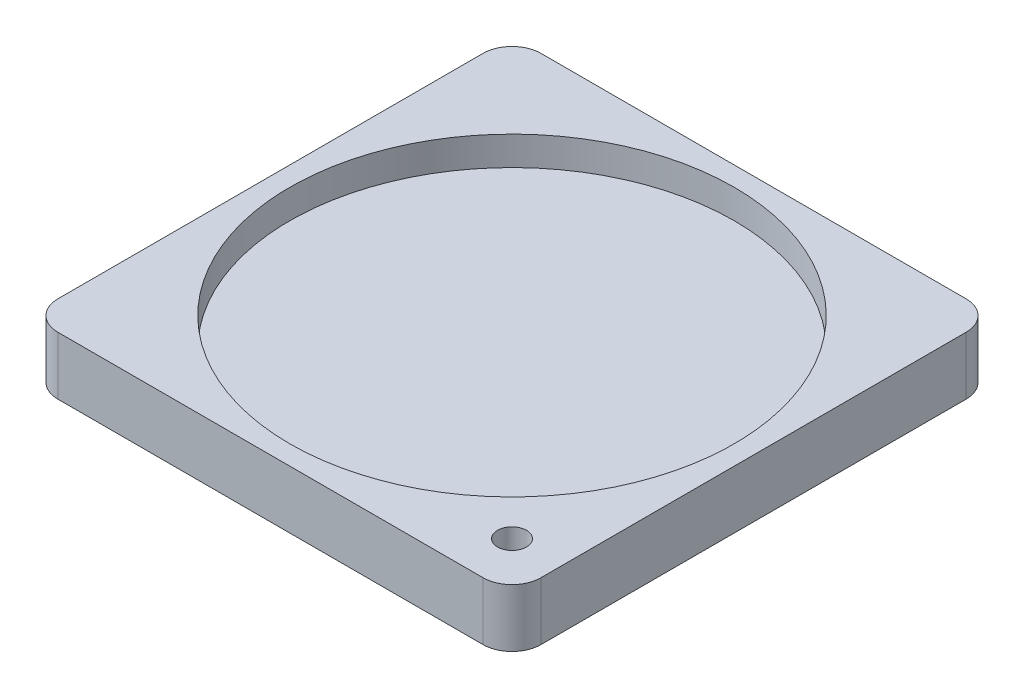
from build123d import *

# Parameters (mm, degrees)
SKETCH1_W           = 50
SKETCH1_H           = 50
BOSS_EXTRUDE1_DEPTH = 10
SKETCH2_R           = 23
CUT_EXTRUDE1_DEPTH  = 3
SKETCH3_R           = 1.5
CUT_EXTRUDE2_DEPTH  = 3
SKETCH4_W           = 50
SKETCH4_H           = 4
CUT_EXTRUDE3_DEPTH  = 76
FILLET1_R           = 3
SKETCH5_R           = 1.5
CUT_EXTRUDE4_DEPTH  = 1


with BuildPart() as part:
    # Sketch1 → Boss-Extrude1 (new body)
    with BuildSketch(Plane(origin=(0, 0, 0), x_dir=(1, 0, 0), z_dir=(0, 1, 0))):
        Rectangle(SKETCH1_W, SKETCH1_H)
    extrude(amount=BOSS_EXTRUDE1_DEPTH)

    # Sketch2 → Cut-Extrude1 (cut)
    with BuildSketch(Plane(origin=(0, 10, 0), x_dir=(1, 0, 0), z_dir=(0, 1, 0))):
        with Locations(Location((0, 0, 0), (0, 0, 270))):
            Circle(SKETCH2_R)
    extrude(amount=-CUT_EXTRUDE1_DEPTH, mode=Mode.SUBTRACT)

    # Sketch3 → Cut-Extrude2 (cut)
    with BuildSketch(Plane(origin=(0, 10, 0), x_dir=(1, 0, 0), z_dir=(0, 1, 0))):
        with Locations(Location((20, -20, 0), (0, 0, 270))):
            Circle(SKETCH3_R)
    extrude(amount=-CUT_EXTRUDE2_DEPTH, mode=Mode.SUBTRACT)

    # Sketch4 → Cut-Extrude3 (cut)
    with BuildSketch(Plane.XY.offset(25)):
        with Locations((0, 2)):
            Rectangle(SKETCH4_W, SKETCH4_H)
    extrude(amount=-CUT_EXTRUDE3_DEPTH, mode=Mode.SUBTRACT)

    # Fillet1
    fillet1_edges = [part.edges().sort_by_distance(p)[0] for p in [
        (25, 7, 25),
        (-25, 7, 25),
        (-25, 7, -25),
        (25, 7, -25),
    ]]
    fillet(fillet1_edges, radius=FILLET1_R)

    # Sketch5 → Cut-Extrude4 (cut)
    with BuildSketch(Plane.XZ.offset(-4)):
        with Locations(Location((-16, 16, 0), (0, 0, 270))):
            Circle(SKETCH5_R)
        with Locations(Location((16, 16, 0), (0, 0, 270))):
            Circle(SKETCH5_R)
        with Locations(Location((-16, -16, 0), (0, 0, 270))):
            Circle(SKETCH5_R)
        with Locations(Location((16, -16, 0), (0, 0, 270))):
            Circle(SKETCH5_R)
    extrude(amount=-CUT_EXTRUDE4_DEPTH, mode=Mode.SUBTRACT)


solid = part.part
